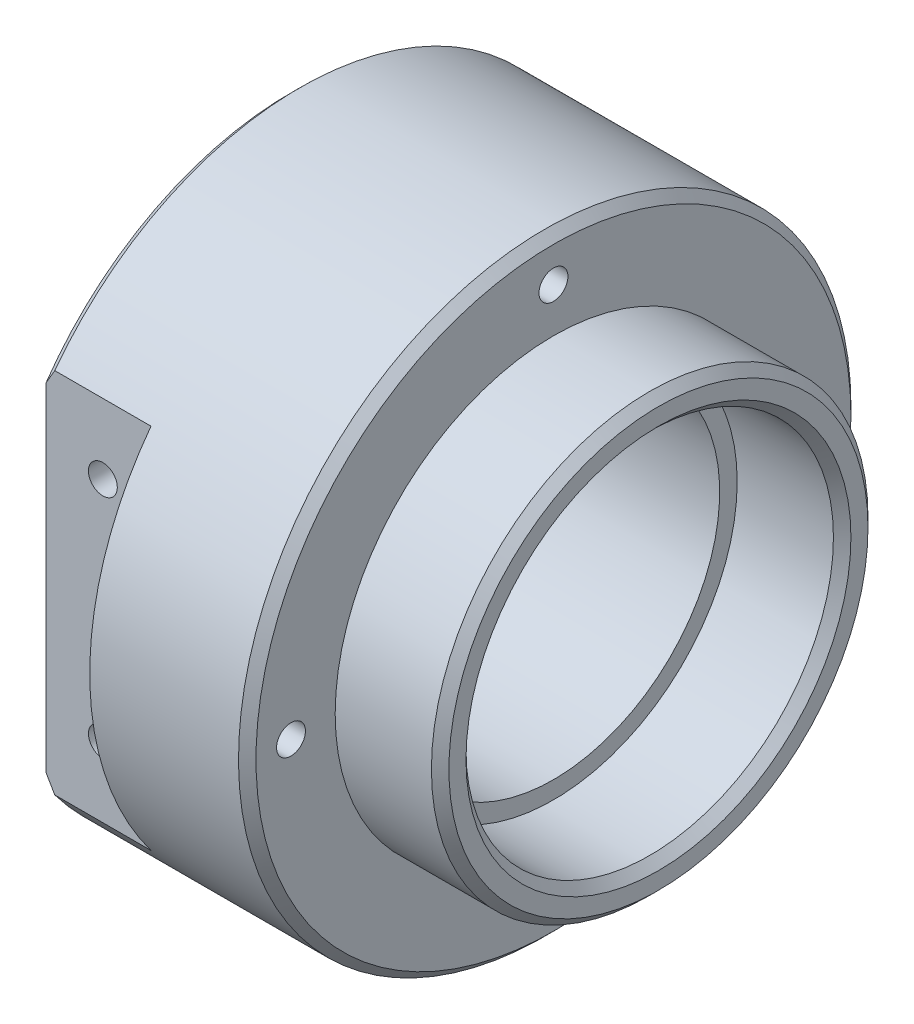
from build123d import *

# Parameters (mm, degrees)
SKETCH1_R             = 35
BOSS_EXTRUDE1_DEPTH   = 20
SKETCH2_R             = 35
BOSS_EXTRUDE2_DEPTH   = 10
SKETCH3_R             = 24.95
BOSS_EXTRUDE3_DEPTH   = 12
SKETCH4_R             = 21
CUT_EXTRUDE1_DEPTH    = 12
SKETCH5_R             = 19
CUT_EXTRUDE2_DEPTH    = 18
SKETCH6_R             = 21
CUT_EXTRUDE3_DEPTH    = 28
CIRPATTERN1_COUNT     = 4
SKETCH9_W             = 82.925750659
SKETCH9_H             = 79.628478102
CUT_EXTRUDE4_DEPTH    = 12
M4_TAPPED_HOLE3_D     = 3.3
M4_TAPPED_HOLE3_DEPTH = 10.1
M4_TAPPED_HOLE3_TIP   = 0.991420021
CHAMFER1_SIZE         = 1


with BuildPart() as part:
    # Sketch1 → Boss-Extrude1 (new body)
    with BuildSketch(Plane(origin=(0, 0, 0), x_dir=(0, 0, -1), z_dir=(1, 0, 0))):
        Circle(SKETCH1_R)
    extrude(amount=BOSS_EXTRUDE1_DEPTH)

    # Sketch2 → Boss-Extrude2 (add)
    with BuildSketch(Plane(origin=(20, 0, 0), x_dir=(0, 0, -1), z_dir=(1, 0, 0))):
        Circle(SKETCH2_R)
    extrude(amount=BOSS_EXTRUDE2_DEPTH)

    # Sketch3 → Boss-Extrude3 (add)
    with BuildSketch(Plane(origin=(30, 0, 0), x_dir=(0, 0, -1), z_dir=(1, 0, 0))):
        Circle(SKETCH3_R)
    extrude(amount=BOSS_EXTRUDE3_DEPTH)

    # Sketch4 → Cut-Extrude1 (cut)
    with BuildSketch(Plane.ZY):
        Circle(SKETCH4_R)
    extrude(amount=-CUT_EXTRUDE1_DEPTH, mode=Mode.SUBTRACT)

    # Sketch5 → Cut-Extrude2 (cut)
    with BuildSketch(Plane.ZY.offset(-12)):
        Circle(SKETCH5_R)
    extrude(amount=-CUT_EXTRUDE2_DEPTH, mode=Mode.SUBTRACT)

    # Sketch6 → Cut-Extrude3 (cut)
    with BuildSketch(Plane.ZY.offset(-30)):
        Circle(SKETCH6_R)
    extrude(amount=-CUT_EXTRUDE3_DEPTH, mode=Mode.SUBTRACT)

    # Sketch7 → M4 Tapped Hole2 (revolve, cut)
    with BuildSketch(Plane(origin=(30, 0, -30), x_dir=(0, 0, -1), z_dir=(0, 1, 0))):
        Polygon((0, 0), (0, 11.091420021), (1.65, 10.1), (1.65, 0), align=None)
    m4_tapped_hole2 = revolve(axis=Axis((36.35, 0, -30), (-1, 0, 0)), mode=Mode.SUBTRACT)

    # CirPattern1: M4 Tapped Hole2 ×4 about axis
    cirpattern1_axis = Axis((0, 0, 0), (1, 0, 0))
    for i in range(1, CIRPATTERN1_COUNT):
        add(m4_tapped_hole2.rotate(cirpattern1_axis, i * 360 / CIRPATTERN1_COUNT), mode=Mode.SUBTRACT)

    # Sketch9 → Cut-Extrude4 (cut)
    with BuildSketch(Plane.ZY):
        with Locations((69.46287533, 0)):
            Rectangle(SKETCH9_W, SKETCH9_H)
    extrude(amount=-CUT_EXTRUDE4_DEPTH, mode=Mode.SUBTRACT)

    # M4 Tapped Hole3
    with Locations(Plane.XY.offset(28)):
        with Locations((6.5, 13), (6.5, -13)):
            Hole(M4_TAPPED_HOLE3_D / 2, depth=M4_TAPPED_HOLE3_DEPTH)
            with Locations((0, 0, -(M4_TAPPED_HOLE3_DEPTH + M4_TAPPED_HOLE3_TIP / 2))):  # 118° drill point
                Cone(0, M4_TAPPED_HOLE3_D / 2, M4_TAPPED_HOLE3_TIP, mode=Mode.SUBTRACT)

    # Chamfer1
    chamfer1_edges = [part.edges().sort_by_distance(p)[0] for p in [
        (42, 0, 24.95),
        (0, 0, -21),
        (42, 0, -21),
        (0, 33.203915432, -11.067971811),
        (30, 0, 35),
    ]]
    chamfer(chamfer1_edges, length=CHAMFER1_SIZE)


solid = part.part
